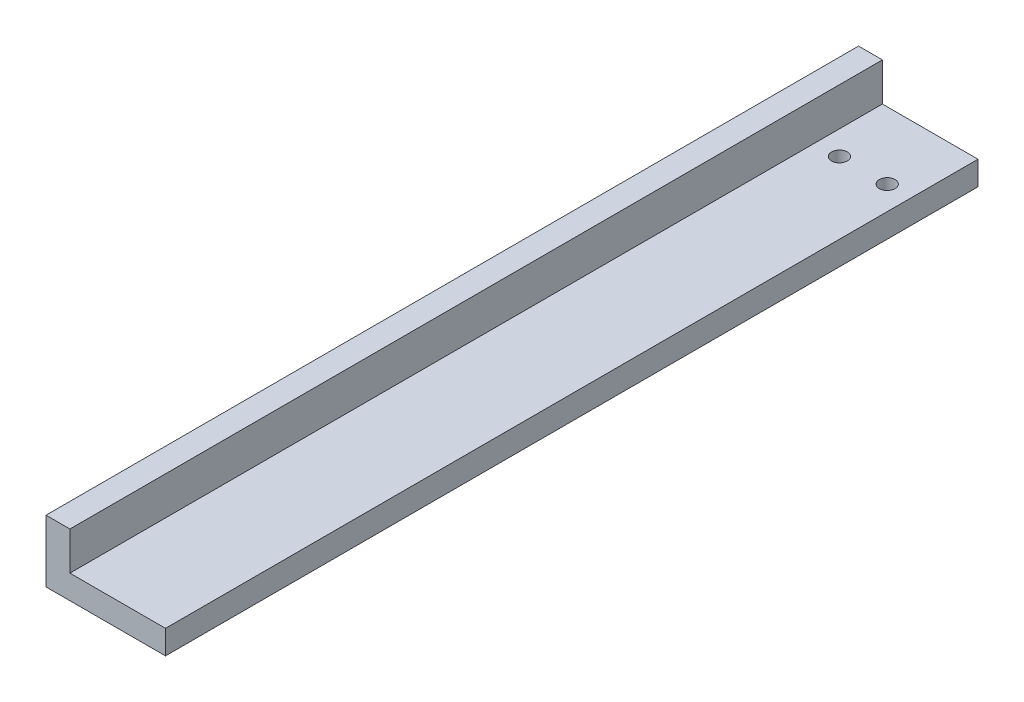
from build123d import *

# Parameters (mm, degrees)
EXTRUDE_1_DEPTH              = 170
HOLE_WIZARD_M4_1_D           = 3.3
HOLE_WIZARD_M4_1_CSINK_D     = 4.05
HOLE_WIZARD_M4_1_CSINK_ANGLE = 90


with BuildPart() as part:
    # 草图1 → 凸台-拉伸1 (new body)
    with BuildSketch(Plane.XY):
        Polygon((0, 0), (0, 13), (5, 13), (5, 5), (25, 5), (25, 0), align=None)
    extrude(amount=EXTRUDE_1_DEPTH)

    # M4 螺纹孔1 (through all)
    with Locations(Plane(origin=(10, 0, 14), x_dir=(-1, 0, 0), z_dir=(0, -1, 0))):
        with Locations((0, 0), (-10, 0)):
            CounterSinkHole(HOLE_WIZARD_M4_1_D / 2, HOLE_WIZARD_M4_1_CSINK_D / 2, counter_sink_angle=HOLE_WIZARD_M4_1_CSINK_ANGLE)


solid = part.part
